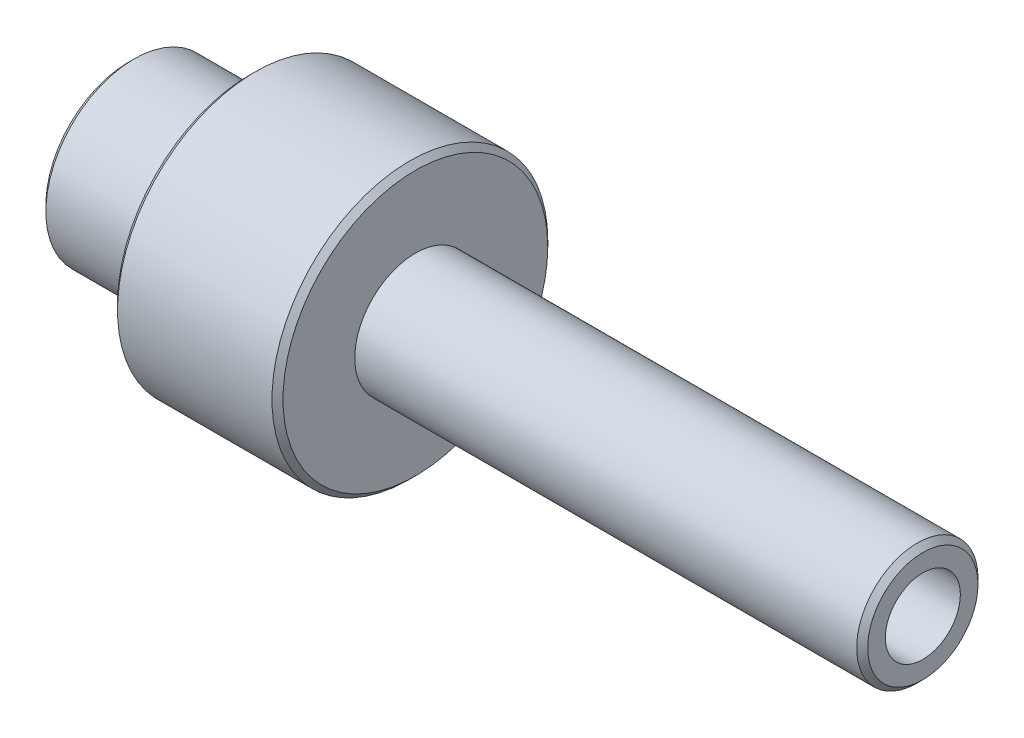
from build123d import *

# Parameters (mm, degrees)
SKETCH1_R             = 8
BOSS_EXTRUDE1_DEPTH   = 11
SKETCH2_R             = 12.5
BOSS_EXTRUDE2_DEPTH   = 15
SKETCH3_R             = 5.5
BOSS_EXTRUDE3_DEPTH   = 46
SKETCH5_R             = 5.5
CUT_EXTRUDE1_DEPTH    = 11
CUT_EXTRUDE2_START    = -2.7
SKETCH6_R             = 6
CUT_EXTRUDE2_DEPTH    = 1.1
SKETCH7_R             = 5
CUT_EXTRUDE3_DEPTH    = 10.2
SKETCH8_R             = 3
CUT_EXTRUDE4_DEPTH    = 15
M8_TAPPED_HOLE1_D     = 6.8
M8_TAPPED_HOLE1_DEPTH = 11
M8_TAPPED_HOLE1_TIP   = 2.042926105
BOSS_EXTRUDE4_START   = -16
SKETCH11_R            = 5.5
BOSS_EXTRUDE4_DEPTH   = 5
SKETCH12_R            = 2.75
CUT_EXTRUDE5_DEPTH    = 5
SKETCH13_R            = 1.5
CUT_EXTRUDE6_DEPTH    = 88
CHAMFER1_SIZE         = 0.5


with BuildPart() as part:
    # Sketch1 → Boss-Extrude1 (new body)
    with BuildSketch(Plane(origin=(0, 0, 0), x_dir=(0, 0, -1), z_dir=(1, 0, 0))):
        Circle(SKETCH1_R)
    extrude(amount=BOSS_EXTRUDE1_DEPTH)

    # Sketch2 → Boss-Extrude2 (add)
    with BuildSketch(Plane(origin=(11, 0, 0), x_dir=(0, 0, -1), z_dir=(1, 0, 0))):
        Circle(SKETCH2_R)
    extrude(amount=BOSS_EXTRUDE2_DEPTH)

    # Sketch3 → Boss-Extrude3 (add)
    with BuildSketch(Plane(origin=(26, 0, 0), x_dir=(0, 0, -1), z_dir=(1, 0, 0))):
        Circle(SKETCH3_R)
    extrude(amount=BOSS_EXTRUDE3_DEPTH)

    # Sketch5 → Cut-Extrude1 (cut)
    with BuildSketch(Plane.ZY):
        with Locations(Location((0, 0, 0), (0, 0, 180))):
            Circle(SKETCH5_R)
    extrude(amount=-CUT_EXTRUDE1_DEPTH, mode=Mode.SUBTRACT)

    # Sketch6 → Cut-Extrude2 (cut)
    with BuildSketch(Plane.ZY.offset(CUT_EXTRUDE2_START)):
        Circle(SKETCH6_R)
    extrude(amount=-CUT_EXTRUDE2_DEPTH, mode=Mode.SUBTRACT)

    # Sketch7 → Cut-Extrude3 (cut)
    with BuildSketch(Plane.ZY.offset(-3.8)):
        Circle(SKETCH7_R)
    extrude(amount=-CUT_EXTRUDE3_DEPTH, mode=Mode.SUBTRACT)

    # Sketch8 → Cut-Extrude4 (cut)
    with BuildSketch(Plane.ZY.offset(-14)):
        Circle(SKETCH8_R)
    extrude(amount=-CUT_EXTRUDE4_DEPTH, mode=Mode.SUBTRACT)

    # M8 Tapped Hole1
    with Locations(Plane(origin=(72, 0, 0), x_dir=(0, 0, -1), z_dir=(1, 0, 0))):
        with Locations((0, 0)):
            Hole(M8_TAPPED_HOLE1_D / 2, depth=M8_TAPPED_HOLE1_DEPTH)
            with Locations((0, 0, -(M8_TAPPED_HOLE1_DEPTH + M8_TAPPED_HOLE1_TIP / 2))):  # 118° drill point
                Cone(0, M8_TAPPED_HOLE1_D / 2, M8_TAPPED_HOLE1_TIP, mode=Mode.SUBTRACT)

    # Sketch11 → Boss-Extrude4 (add)
    with BuildSketch(Plane(origin=(72, 0, 0), x_dir=(0, 0, -1), z_dir=(1, 0, 0)).offset(BOSS_EXTRUDE4_START)):
        Circle(SKETCH11_R)
    extrude(amount=BOSS_EXTRUDE4_DEPTH)

    # Sketch12 → Cut-Extrude5 (cut)
    with BuildSketch(Plane(origin=(61, 0, 0), x_dir=(0, 0, -1), z_dir=(1, 0, 0))):
        Circle(SKETCH12_R)
    extrude(amount=-CUT_EXTRUDE5_DEPTH, mode=Mode.SUBTRACT)

    # Sketch13 → Cut-Extrude6 (cut)
    with BuildSketch(Plane(origin=(56, 0, 0), x_dir=(0, 0, -1), z_dir=(1, 0, 0))):
        Circle(SKETCH13_R)
    extrude(amount=-CUT_EXTRUDE6_DEPTH, mode=Mode.SUBTRACT)

    # Chamfer1
    chamfer1_edges = [part.edges().sort_by_distance(p)[0] for p in [
        (72, 0, 5.5),
        (0, 0, 8),
        (11, 0, 12.5),
        (26, 0, 12.5),
    ]]
    chamfer(chamfer1_edges, length=CHAMFER1_SIZE)


solid = part.part
